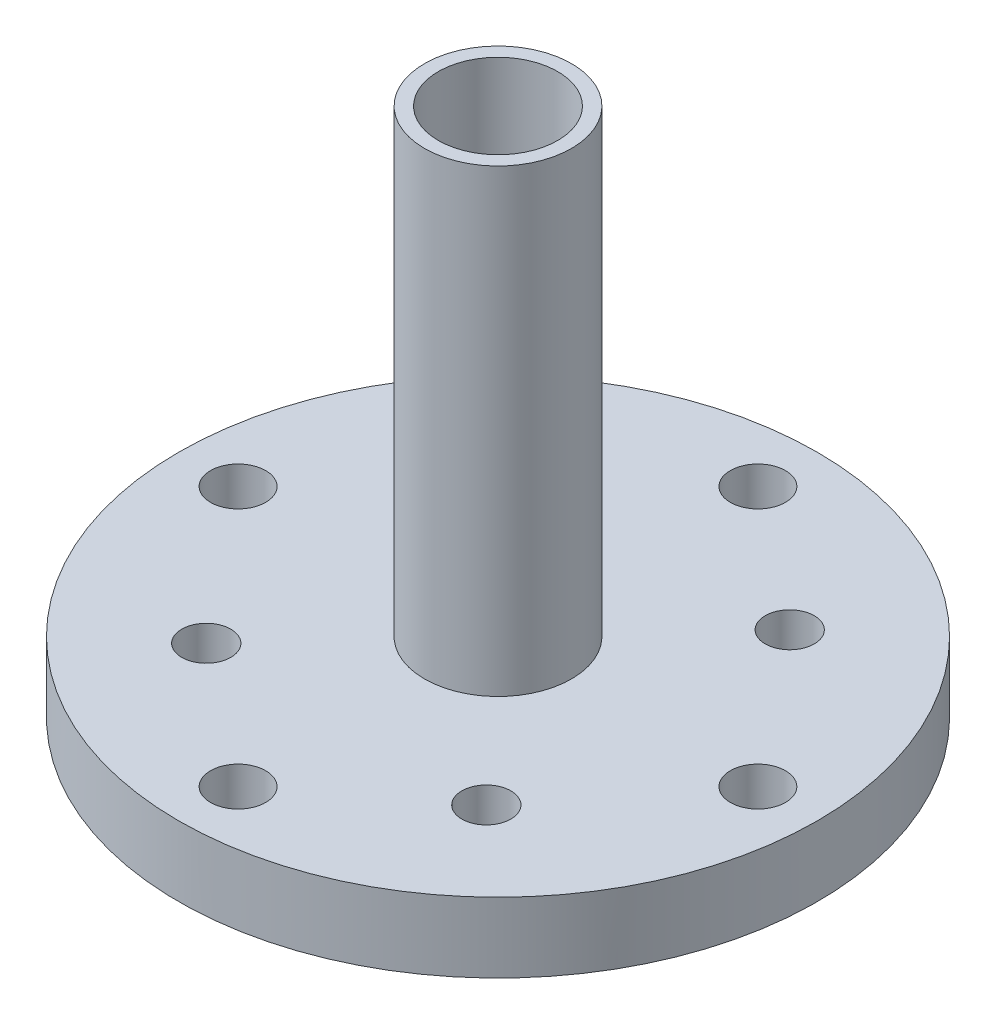
SolidWorks part; units mm, degrees
ref_plane "Front Plane" through (0, 0, 0) normal (0, 0, 1) x (1, 0, 0)
ref_plane "Top Plane" through (0, 0, 0) normal (0, 1, 0) x (1, 0, 0)
ref_plane "Right Plane" through (0, 0, 0) normal (1, 0, 0) x (0, 0, -1)
sketch "Sketch1" plane through (0, 0, 0) normal (0, 1, 0) x (1, 0, 0)
  line L0 (-45.4279, 0) -> (86.5356, 0) construction
  line L1 (0, 55.7505) -> (0, -37.9378) construction
  circle A0 centre (0, 0) radius 31.75
  circle A1 centre (-15.24, 16.51) radius 2.667
  circle A2 centre (15.24, 16.51) radius 2.667
  circle A3 centre (15.24, -16.51) radius 2.667
  circle A4 centre (-15.24, -16.51) radius 2.667
  dimension "D1" = 63.5
  dimension "D2" = 5.334
  dimension "D3" = 5.334
  dimension "D4" = 5.334
  dimension "D5" = 5.334
  dimension "D8" = 15.24
  dimension "D13" = 16.51
  dimension "D6" = 15.24
  dimension "D7" = 15.24
  dimension "D9" = 15.24
  dimension "D10" = 16.51
  dimension "D11" = 16.51
  dimension "D12" = 16.51
extrude "Boss-Extrude1" add sketch "Sketch1" against normal blind 7.62
sketch "Sketch2" plane through (0, 0, 0) normal (0, 1, 0) x (1, 0, 0)
  circle A0 centre (0, 0) radius 6.604
  dimension "D1" = 13.208
extrude "Cut-Extrude1" cut sketch "Sketch2" against normal through all
sketch "草图1" plane through (0, -7.62, 0) normal (0, -1, 0) x (1, 0, 0)
  circle A0 centre (0, 0) radius 7.5
  dimension "D1" = 15
extrude "凸台-拉伸1" add sketch "草图1" against normal up to surface (7.62 mm away) up to face at (0, 0, 6.604)
sketch "草图2" plane through (0, 0, 0) normal (0, 1, 0) x (1, 0, 0)
  circle A0 centre (0, 0) radius 6.5
  circle A1 centre (0, 0) radius 8
  dimension "D1" = 13
  dimension "D2" = 16
extrude "Boss-Extrude2" add sketch "草图2" along normal blind 50
scale "Scale1" bodies to scale 105 scale about origin uniform scaling yes scale factor 2
sketch "Sketch3" plane through (0, 0, 0) normal (0, 1, 0) x (1, 0, 0)
  line L0 (-56.5685, 0) -> (0, 56.5685) construction
  line L1 (-56.5685, 0) -> (0, -56.5685) construction
  line L2 (0, 56.5685) -> (56.5685, 0) construction
  line L3 (0, -56.5685) -> (56.5685, 0) construction
  line L4 (-56.5685, 0) -> (56.5685, 0) construction
  line L5 (0, 56.5685) -> (0, -56.5685) construction
  circle A2 centre (56.5685, 0) radius 6
  circle A3 centre (0, -56.5685) radius 6
  circle A4 centre (-56.5685, 0) radius 6
  circle A5 centre (0, 56.5685) radius 6
  point P15 (0, 0)
  dimension "D2" = 12
  dimension "D4" = 80
  dimension "D3" = 4
extrude "切除-拉伸1" cut sketch "Sketch3" against normal blind 21
sketch "Sketch5" plane through (0, -15.24, 0) normal (0, -1, 0) x (1, 0, 0)
  circle A0 centre (0, 0) radius 69.5
  circle A2 centre (0, 0) radius 63.5
  circle A3 centre (0, 0) radius 63.5
  dimension "D1" = 139
  dimension "D2" = 0
extrude "Boss-Extrude3" add sketch "Sketch5" against normal up to surface (15.24 mm away) up to face at (56.5685, 0, 6)
